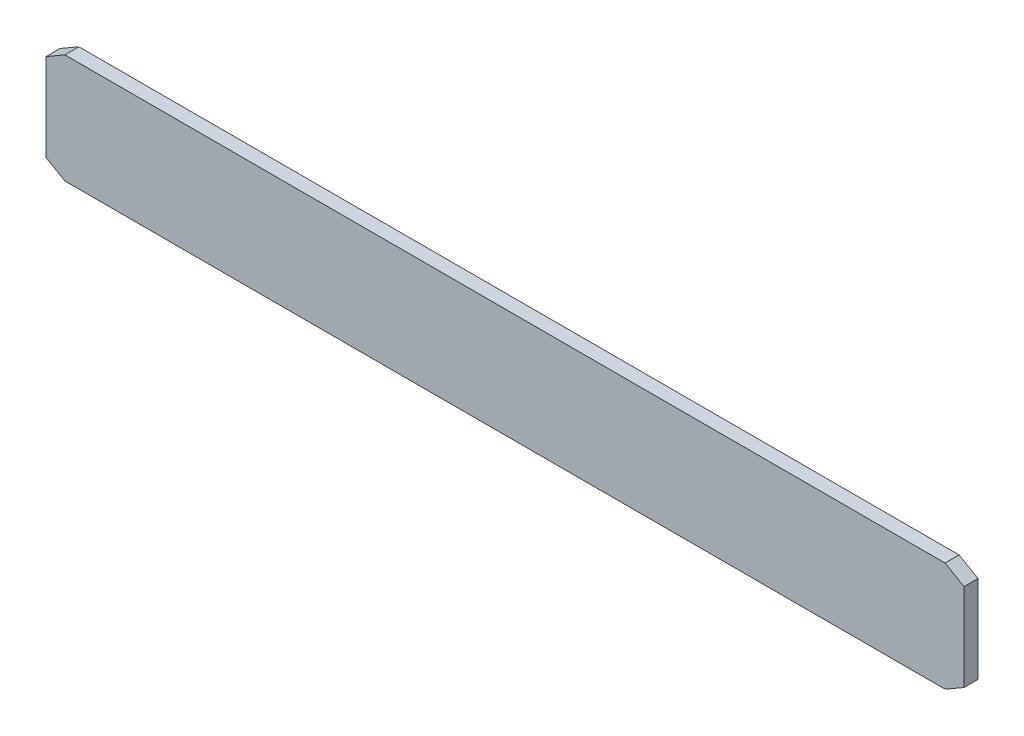
from build123d import *

# Parameters (mm, degrees)
BOSS_EXTRUDE1_DEPTH = 16


with BuildPart() as part:
    # Sketch1 → Boss-Extrude1 (new, symmetric)
    with BuildSketch(Plane.XY):
        Polygon((1050, 100), (1006.698729811, 125), (-1006.698729811, 125), (-1050, 100), (-1050, -100), (-1006.698729811, -125), (1006.698729811, -125), (1050, -100), align=None)
    extrude(amount=BOSS_EXTRUDE1_DEPTH, both=True)


solid = part.part
